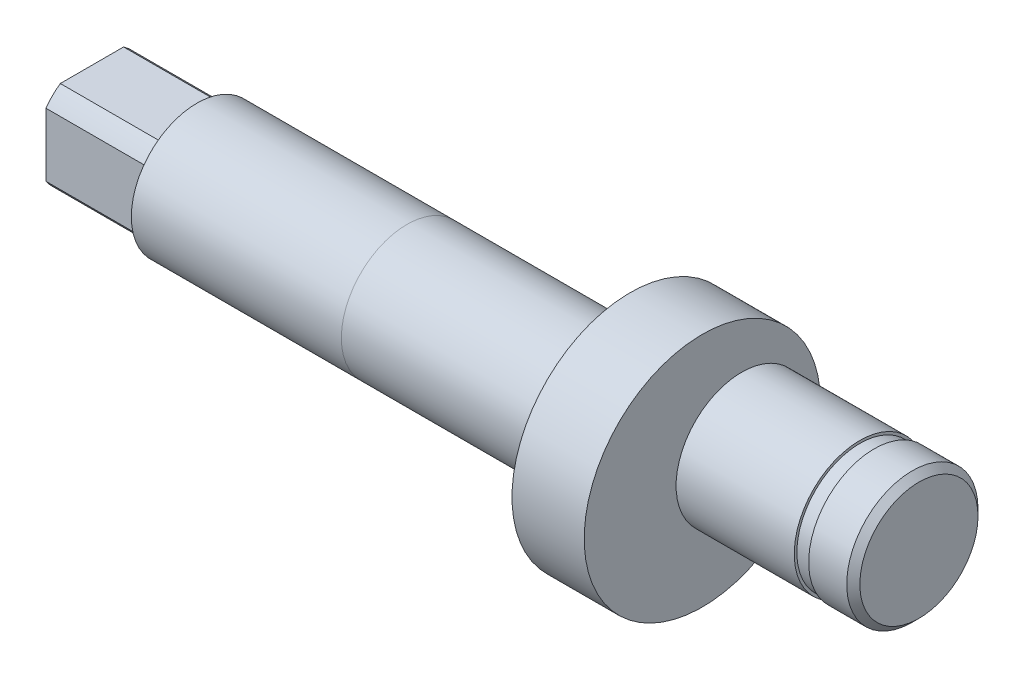
SolidWorks part; units mm, degrees
ref_plane "前视基准面" through (0, 0, 0) normal (0, 0, 1) x (1, 0, 0)
ref_plane "上视基准面" through (0, 0, 0) normal (0, 1, 0) x (1, 0, 0)
ref_plane "右视基准面" through (0, 0, 0) normal (1, 0, 0) x (0, 0, -1)
other "Configuration Table"
sketch "草图2" plane through (0, 0, 0) normal (1, 0, 0) x (0, 0, -1)
  circle A0 centre (0, 0) radius 9
  dimension "D1" = 18
extrude "凸台-拉伸1" add sketch "草图2" along normal blind 5.5
sketch "草图3" plane through (5.5, 0, 0) normal (1, 0, 0) x (0, 0, -1)
  circle A0 centre (3, 0) radius 5
  dimension "D1" = 10
  dimension "D2" = 3
extrude "凸台-拉伸2" add sketch "草图3" along normal blind 9
sketch "草图4" plane through (14.5, 0, 0) normal (1, 0, 0) x (0, 0, -1)
  circle A0 centre (3, 0) radius 4.8
  dimension "D1" = 9.6
extrude "凸台-拉伸3" add sketch "草图4" along normal blind 1.1
sketch "草图5" plane through (15.6, 0, 0) normal (1, 0, 0) x (0, 0, -1)
  circle A0 centre (3, 0) radius 5
  dimension "D1" = 10
extrude "凸台-拉伸4" add sketch "草图5" along normal blind 3.4
chamfer "倒角1" distance 0.5 angle 45 1 edges at (19, 0, -8)
sketch "草图6" plane through (0, 0, 0) normal (-1, 0, 0) x (0, 0, 1)
  circle A0 centre (0, 0) radius 5
  dimension "D1" = 10
extrude "凸台-拉伸5" add sketch "草图6" along normal blind 17
sketch "草图7" plane through (-17, 0, 0) normal (-1, 0, 0) x (0, 0, 1)
  circle A0 centre (0, 0) radius 5
  dimension "D1" = 10
extrude "凸台-拉伸6" add sketch "草图7" along normal blind 16 separate body
cosmetic thread "装饰螺纹线1" parameters "D2"=8.376
sketch "草图8" plane through (-33, 0, 0) normal (-1, 0, 0) x (0, 0, 1)
  line L1 (-2.4109, -3.5) -> (2.4109, -3.5)
  line L2 (-3.5, -2.4109) -> (-3.5, 2.4109)
  line L3 (-2.4109, 3.5) -> (2.4109, 3.5)
  line L4 (3.5, -2.4109) -> (3.5, 2.4109)
  line L5 (0, 3.5) -> (0, -3.5) construction
  line L6 (-3.5, 0) -> (3.5, 0) construction
  arc A0 (-2.4109, 3.5) -> (-3.5, 2.4109) centre (0, 0) ccw
  arc A1 (-3.5, -2.4109) -> (-2.4109, -3.5) centre (0, 0) ccw
  arc A2 (2.4109, -3.5) -> (3.5, -2.4109) centre (0, 0) ccw
  arc A3 (3.5, 2.4109) -> (2.4109, 3.5) centre (0, 0) ccw
  point P0 (0, 0)
  dimension "D1" = 8.5
  dimension "D3" = 3.5
  dimension "D2" = 7
  dimension "D4" = 3.5
extrude "凸台-拉伸7" add sketch "草图8" along normal blind 8
